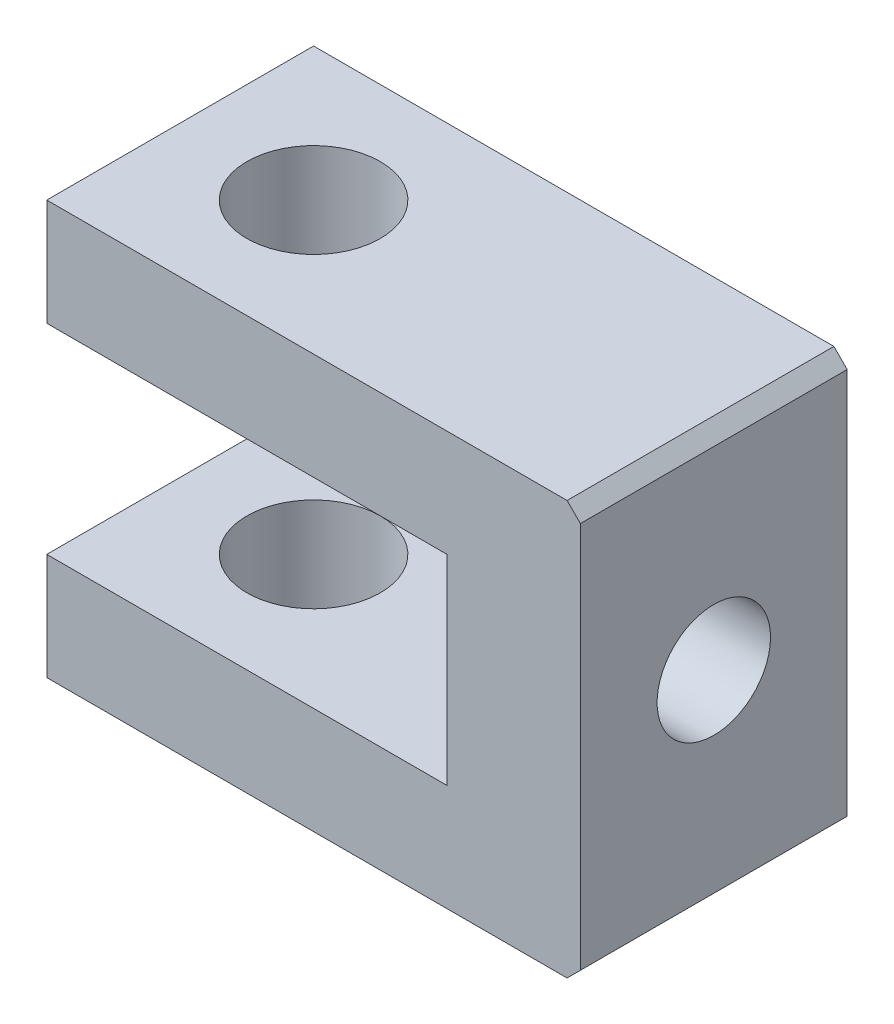
SolidWorks part; units mm, degrees
ref_plane "前视基准面" through (0, 0, 0) normal (0, 0, 1) x (1, 0, 0)
ref_plane "上视基准面" through (0, 0, 0) normal (0, 1, 0) x (1, 0, 0)
ref_plane "右视基准面" through (0, 0, 0) normal (1, 0, 0) x (0, 0, -1)
ref_plane "基准面4" through (0, 0, -10) normal (0, 0, -1) x (-1, 0, 0)
sketch "草图1" plane through (0, 0, -10) normal (0, 0, -1) x (-1, 0, 0)
  line L0 (16.9616, -15.5) -> (16.9616, 15.5)
  line L1 (16.9616, 15.5) -> (-23.0384, 15.5)
  line L2 (-23.0384, 15.5) -> (-23.0384, -15.5)
  line L3 (-23.0384, -15.5) -> (16.9616, -15.5)
extrude "凸台-拉伸1" add sketch "草图1" against normal blind 20
sketch "草图2" plane through (0, 0, 10) normal (0, 0, 1) x (1, 0, 0)
  line L0 (-16.9616, 7.5) -> (-16.9616, -7.5)
  line L1 (-16.9616, -7.5) -> (13.0384, -7.5)
  line L2 (13.0384, -7.5) -> (13.0384, 7.5)
  line L3 (13.0384, 7.5) -> (-16.9616, 7.5)
extrude "切除-拉伸1" cut sketch "草图2" against normal through all
hole_wizard "Ø10.0 (10) 直径孔1" positions "草图4" profile "草图3" hole size "Ø10.0" standard "ANSI Metric"
sketch "草图4" plane through (0, -15.5, 0) normal (0, -1, 0) x (-1, 0, 0)
  point P0 (6.9616, 0)
sketch "草图3" plane through (-6.9616, -15.5, 0) normal (1, 0, 0) x (0, 0, -1)
  line L0 (0, 0) -> (0, 8)
  line L1 (0, 8) -> (5, 8)
  line L2 (5, 8) -> (5, 0)
  line L5 (5, 0) -> (0, 0)
  line L11 (0, -6.35) -> (0, 107.95) construction
  dimension "通孔孔直径" = 10
  dimension "通孔孔深度" = 8
hole_wizard "Ø8.5 (8.5) 直径孔1" positions "草图6" profile "草图5" hole size "Ø8.5" standard "ANSI Metric"
sketch "草图6" plane through (23.0384, 0, 0) normal (1, 0, 0) x (0, 0, -1)
  point P0 (0, 0)
sketch "草图5" plane through (23.0384, 0, 0) normal (0, 1, 0) x (0, 0, -1)
  line L0 (0, 0) -> (0, 40)
  line L1 (0, 40) -> (4.25, 40)
  line L2 (4.25, 40) -> (4.25, 0)
  line L5 (4.25, 0) -> (0, 0)
  line L11 (0, -6.35) -> (0, 107.95) construction
  dimension "通孔孔直径" = 8.5
  dimension "通孔孔深度" = 40
hole_wizard "Ø10.0 (10) 直径孔2" positions "草图8" profile "草图7" hole size "Ø10.0" standard "ANSI Metric"
sketch "草图8" plane through (0, 7.5, 0) normal (0, -1, 0) x (-1, 0, 0)
  point P0 (6.9616, 0)
sketch "草图7" plane through (-6.9616, 7.5, 0) normal (1, 0, 0) x (0, 0, -1)
  line L0 (0, 0) -> (0, 8)
  line L1 (0, 8) -> (5, 8)
  line L2 (5, 8) -> (5, 0)
  line L5 (5, 0) -> (0, 0)
  line L11 (0, -6.35) -> (0, 107.95) construction
  dimension "通孔孔直径" = 10
  dimension "通孔孔深度" = 8
chamfer "倒角1" distance 1 angle 45 2 edges at (23.0384, 15.5, 0) (23.0384, -15.5, 0)
